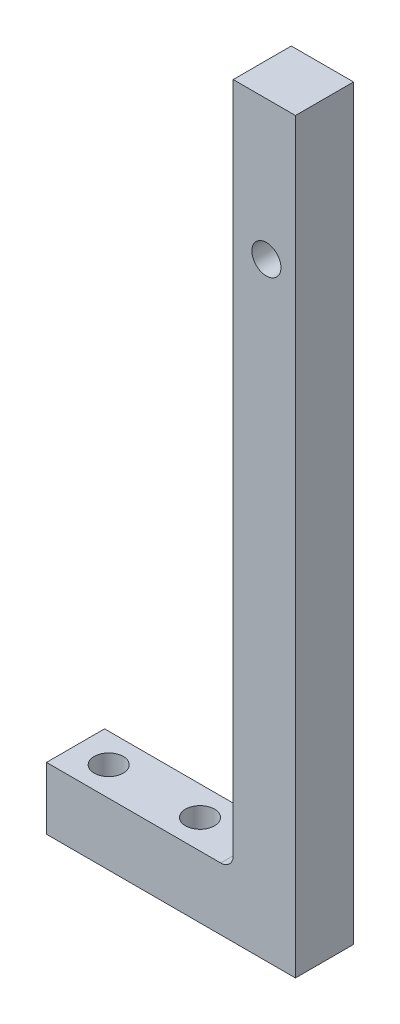
from build123d import *

# Parameters (mm, degrees)
EXTRUDE_1_DEPTH     = 7
FILLET_1_R          = 3
CUT_EXTRUDE_1_REACH = 177.71
SKETCH_3_R          = 3.5
CUT_EXTRUDE_2_REACH = 192.252
SKETCH_4_R          = 3.5


with BuildPart() as part:
    # 草图1 → 凸台-拉伸1 (new, symmetric)
    with BuildSketch(Plane.XY):
        Polygon((0, 180), (-15, 180), (-15, 15), (-60, 15), (-60, 0), (0, 0), align=None)
    extrude(amount=EXTRUDE_1_DEPTH, both=True)

    # 圆角1
    fillet_1_edges = [part.edges().sort_by_distance(p)[0] for p in [
        (-15, 15, 0),
    ]]
    fillet(fillet_1_edges, radius=FILLET_1_R)

    # 草图3 → 切除-拉伸1 (cut, up to next)
    with BuildSketch(Plane(origin=(0, 15, 0), x_dir=(1, 0, 0), z_dir=(0, 1, 0)), mode=Mode.PRIVATE) as cut_extrude_1_sk1:
        with Locations(Location((-52, 0, 0), (0, 0, 180))):
            Circle(SKETCH_3_R)
    cut_extrude_1_tool1 = extrude(cut_extrude_1_sk1.sketch, amount=-CUT_EXTRUDE_1_REACH, mode=Mode.PRIVATE) & part.part
    # 草图3 → 切除-拉伸1 (cut, up to next)
    with BuildSketch(Plane(origin=(0, 15, 0), x_dir=(1, 0, 0), z_dir=(0, 1, 0)), mode=Mode.PRIVATE) as cut_extrude_1_sk2:
        with Locations(Location((-30, 0, 0), (0, 0, 180))):
            Circle(SKETCH_3_R)
    cut_extrude_1_tool2 = extrude(cut_extrude_1_sk2.sketch, amount=-CUT_EXTRUDE_1_REACH, mode=Mode.PRIVATE) & part.part
    add(cut_extrude_1_tool1.solids().sort_by_distance((-52, 15, 0))[0], mode=Mode.SUBTRACT)
    add(cut_extrude_1_tool2.solids().sort_by_distance((-30, 15, 0))[0], mode=Mode.SUBTRACT)

    # 草图4 → 切除-拉伸2 (cut, up to next)
    with BuildSketch(Plane(origin=(0, 0, -7), x_dir=(-1, 0, 0), z_dir=(0, 0, -1)), mode=Mode.PRIVATE) as cut_extrude_2_sk1:
        with Locations((7, 146.5)):
            Circle(SKETCH_4_R)
    cut_extrude_2_tool1 = extrude(cut_extrude_2_sk1.sketch, amount=-CUT_EXTRUDE_2_REACH, mode=Mode.PRIVATE) & part.part
    add(cut_extrude_2_tool1.solids().sort_by_distance((-7, 146.5, -7))[0], mode=Mode.SUBTRACT)


solid = part.part
